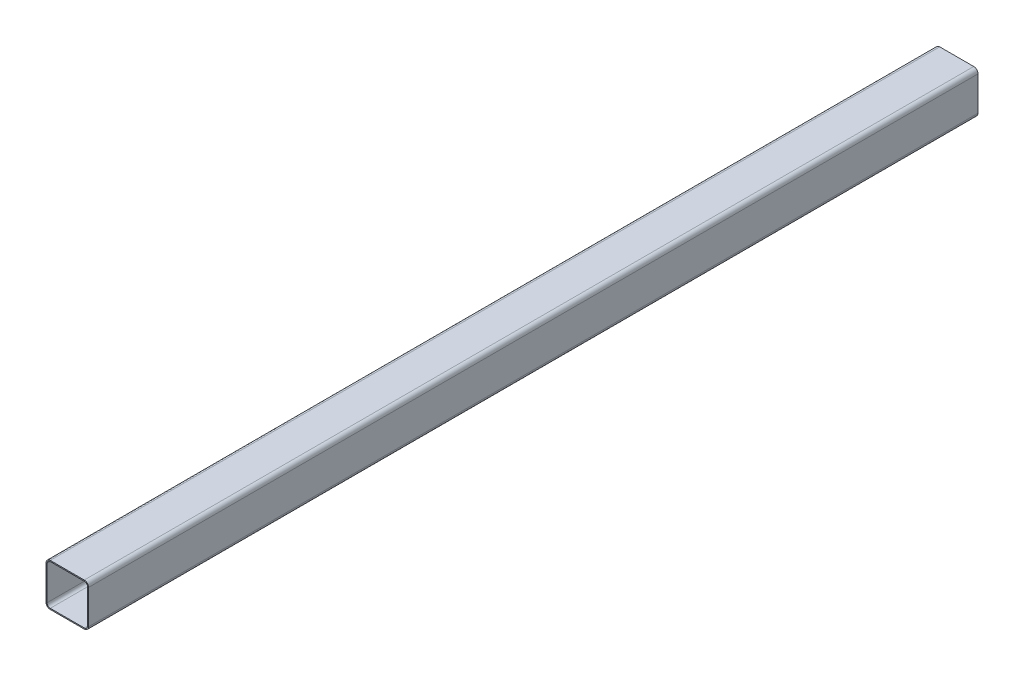
SolidWorks part; units mm, degrees
ref_plane "Front Plane" through (0, 0, 0) normal (0, 0, 1) x (1, 0, 0)
ref_plane "Top Plane" through (0, 0, 0) normal (0, 1, 0) x (1, 0, 0)
ref_plane "Right Plane" through (0, 0, 0) normal (1, 0, 0) x (0, 0, -1)
other "Configuration Table"
sketch "Sketch1" plane through (0, 0, 0) normal (0, 0, 1) x (1, 0, 0)
  line L0 (-95, 80) -> (-95, -80)
  line L1 (-80, 100) -> (80, 100)
  line L2 (-100, 80) -> (-100, -80)
  line L3 (-80, -100) -> (80, -100)
  line L4 (100, 80) -> (100, -80)
  line L5 (-100, 100) -> (100, -100) construction
  line L6 (-100, -100) -> (100, 100) construction
  line L7 (-80, -95) -> (80, -95)
  line L8 (95, 80) -> (95, -80)
  line L9 (-80, 95) -> (80, 95)
  arc A0 (-100, -80) -> (-80, -100) centre (-80, -80) ccw
  arc A1 (80, -100) -> (100, -80) centre (80, -80) ccw
  arc A2 (80, 100) -> (100, 80) centre (80, 80) cw
  arc A3 (-80, 100) -> (-100, 80) centre (-80, 80) ccw
  arc A4 (-95, -80) -> (-80, -95) centre (-80, -80) ccw
  arc A5 (80, -95) -> (95, -80) centre (80, -80) ccw
  arc A6 (80, 95) -> (95, 80) centre (80, 80) cw
  arc A7 (-80, 95) -> (-95, 80) centre (-80, 80) ccw
  point P0 (0, 0)
  dimension "D3" = 20
  dimension "D1" = 200
  dimension "D2" = 200
  dimension "D4" = 5
extrude "Boss-Extrude1" add sketch "Sketch1" along normal blind 4180
